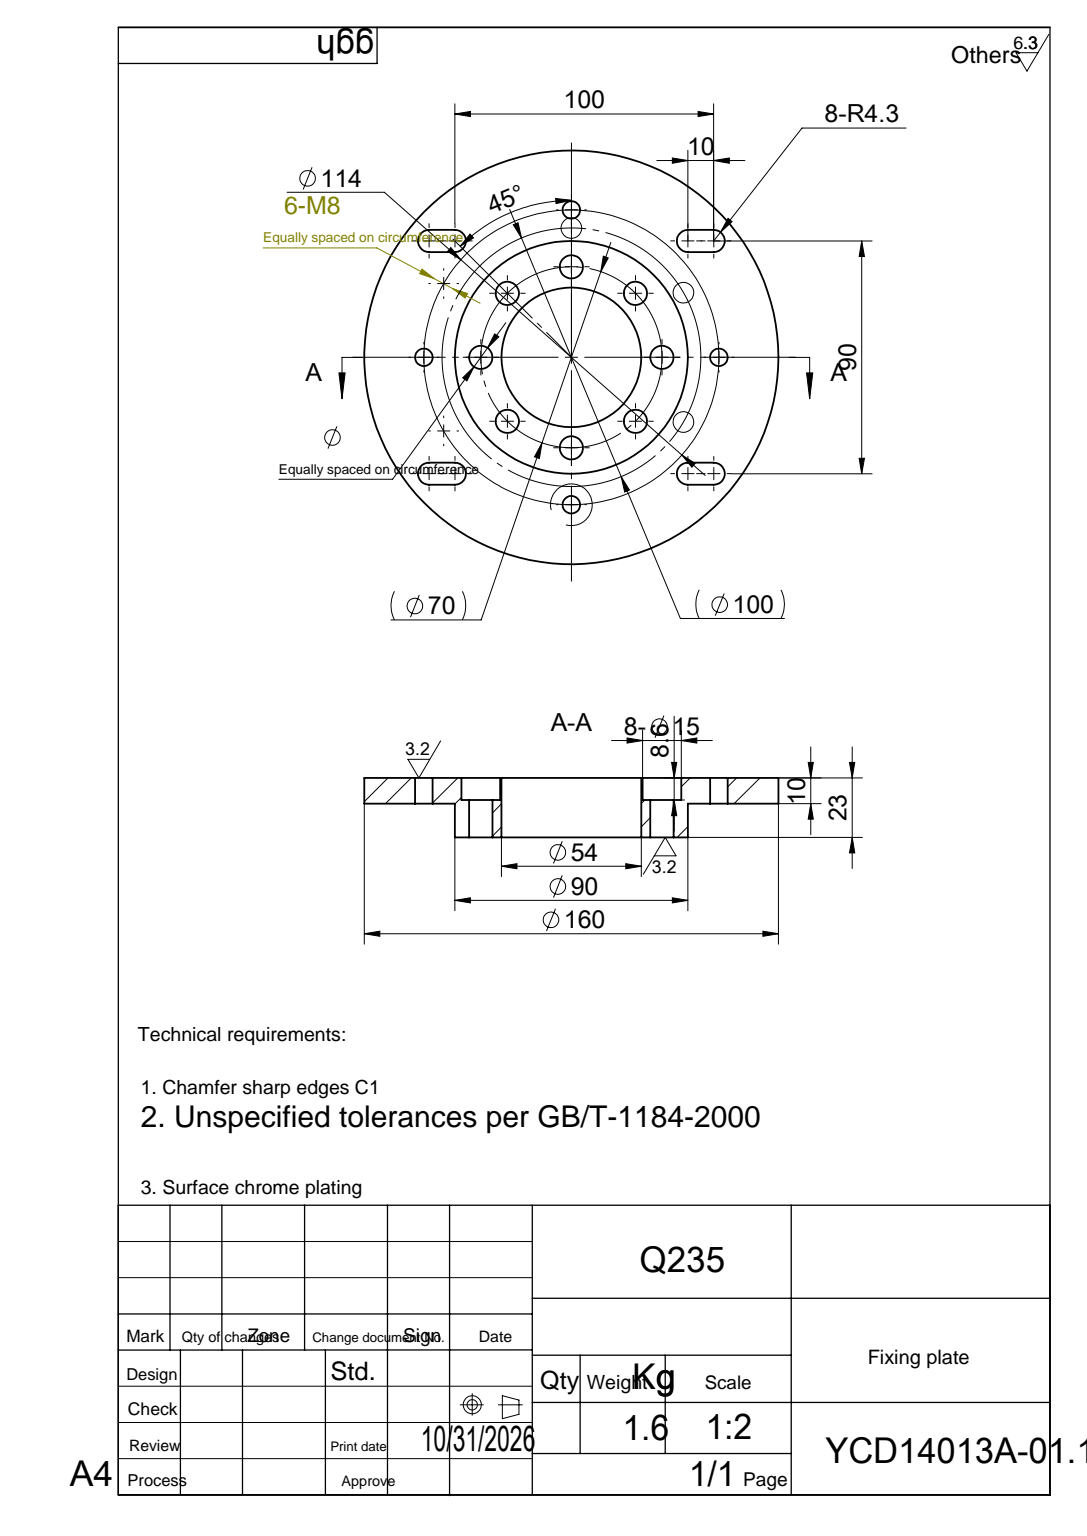
SolidWorks part; units mm, degrees
material "Q235"
ref_plane "Front Plane" through (0, 0, 0) normal (0, 0, 1) x (1, 0, 0)
ref_plane "Top Plane" through (0, 0, 0) normal (0, 1, 0) x (1, 0, 0)
ref_plane "Right Plane" through (0, 0, 0) normal (1, 0, 0) x (0, 0, -1)
sketch "Sketch1" plane through (0, 0, 0) normal (0, 0, 1) x (1, 0, 0)
  circle A0 centre (0, 0) radius 45
  circle A1 centre (0, 0) radius 27
  dimension "D1" = 90
  dimension "D2" = 54
extrude "Boss-Extrude1" add sketch "Sketch1" along normal blind 13
sketch "Sketch2" plane through (0, 0, 0) normal (0, 0, 1) x (1, 0, 0)
  circle A0 centre (0, 0) radius 80
  point P0 (0, 0)
  dimension "D1" = 160
extrude "Boss-Extrude2" add sketch "Sketch2" against normal blind 10
hole_wizard "M8 Tapped Hole1" positions "Sketch4" profile "Sketch3" tap size "M8" standard "Iso"
sketch "Sketch4" plane through (0, 0, 0) normal (0, 0, 1) x (1, 0, 0)
  point P0 (0, -57)
  dimension "D1" = 57
sketch "Sketch3" plane through (0, -57, 0) normal (1, 0, 0) x (0, -1, 0)
  line L0 (0, 0) -> (0, 24.3429)
  line L1 (0, 24.3429) -> (3.4, 22.3)
  line L2 (3.4, 22.3) -> (3.4, 0)
  line L5 (3.4, 0) -> (0, 0)
  line L10 (0, 24.3429) -> (-3.4, 22.3) construction
  line L11 (0, -6.35) -> (0, 107.95) construction
  dimension "螺纹孔钻头直径" = 6.8
  dimension "螺纹孔钻头深度" = 22.3
  dimension "导头角度" = 118
cosmetic thread "Cosmetic Thread1" parameters "D1"=10, "D2"=8
sketch "Sketch5" plane through (0, 0, 0) normal (0, 0, 1) x (1, 0, 0)
  line L0 (45, 45) -> (55, 45) construction
  line L1 (45, 49.2719) -> (55, 49.2719)
  line L2 (45, 40.7281) -> (55, 40.7281)
  line L3 (45, -45) -> (55, -45) construction
  line L4 (45, -40.7281) -> (55, -40.7281)
  line L5 (45, -49.2719) -> (55, -49.2719)
  line L6 (0, 0) -> (86.5049, 0) construction
  line L7 (0, 0) -> (0, 115.3787) construction
  line L8 (-45, -45) -> (-55, -45) construction
  line L9 (-45, -40.7281) -> (-55, -40.7281)
  line L10 (-45, -49.2719) -> (-55, -49.2719)
  line L11 (-45, 45) -> (-55, 45) construction
  line L12 (-45, 49.2719) -> (-55, 49.2719)
  line L13 (-45, 40.7281) -> (-55, 40.7281)
  arc A0 (45, 49.2719) -> (45, 40.7281) centre (45, 45) ccw
  arc A1 (55, 40.7281) -> (55, 49.2719) centre (55, 45) ccw
  arc A2 (45, -40.7281) -> (45, -49.2719) centre (45, -45) ccw
  arc A3 (55, -49.2719) -> (55, -40.7281) centre (55, -45) ccw
  arc A4 (-45, -40.7281) -> (-45, -49.2719) centre (-45, -45) cw
  arc A5 (-55, -49.2719) -> (-55, -40.7281) centre (-55, -45) cw
  arc A6 (-45, 49.2719) -> (-45, 40.7281) centre (-45, 45) cw
  arc A7 (-55, 40.7281) -> (-55, 49.2719) centre (-55, 45) cw
  point P2 (50, 45)
  point P8 (50, -45)
  point P20 (-50, -45)
  point P27 (-50, 45)
  dimension "D1" = 100
  dimension "D2" = 90
  dimension "D3" = 10
  dimension "D4" = 8.5438
extrude "Cut-Extrude1" cut sketch "Sketch5" against normal through all
pattern_circular "CirPattern1" count 4 over 360 about axis through (0, 0, 0) along (0, 0, 1) of "M8 Tapped Hole1"
sketch "Sketch6" plane through (0, 0, 0) normal (0, 0, 1) x (1, 0, 0)
  circle A0 centre (0, 0) radius 27 construction
  circle A1 centre (0, 0) radius 27
extrude "Cut-Extrude2" cut sketch "Sketch6" against normal through all
hole_wizard "CBORE for M8 Hex Socket Head Cap Screw1" positions "Sketch8" profile "Sketch9" counterbore size "M8" standard "Iso" end condition through all
sketch "Sketch8" plane through (0, 0, -10) normal (0, 0, -1) x (-1, 0, 0)
  point P0 (35, 0)
  dimension "D1" = 35
sketch "Sketch9" plane through (-35, 0, -10) normal (1, 0, 0) x (0, 1, 0)
  line L0 (0, 0) -> (0, 23)
  line L1 (0, 23) -> (4.5, 23)
  line L3 (4.5, 23) -> (4.5, 8.6)
  line L4 (4.5, 8.6) -> (7.5, 8.6)
  line L5 (7.5, 8.6) -> (7.5, 0)
  line L7 (7.5, 0) -> (0, 0)
  line L11 (0, -6.35) -> (0, 107.95) construction
  dimension "通孔孔直径" = 9
  dimension "通孔孔深度" = 23
  dimension "柱形沉头孔直径" = 15
  dimension "柱形沉头孔深度" = 8.6
pattern_circular "CirPattern2" count 8 over 360 about axis through (0, 0, 0) along (0, 0, 1) of "CBORE for M8 Hex Socket Head Cap Screw1"
